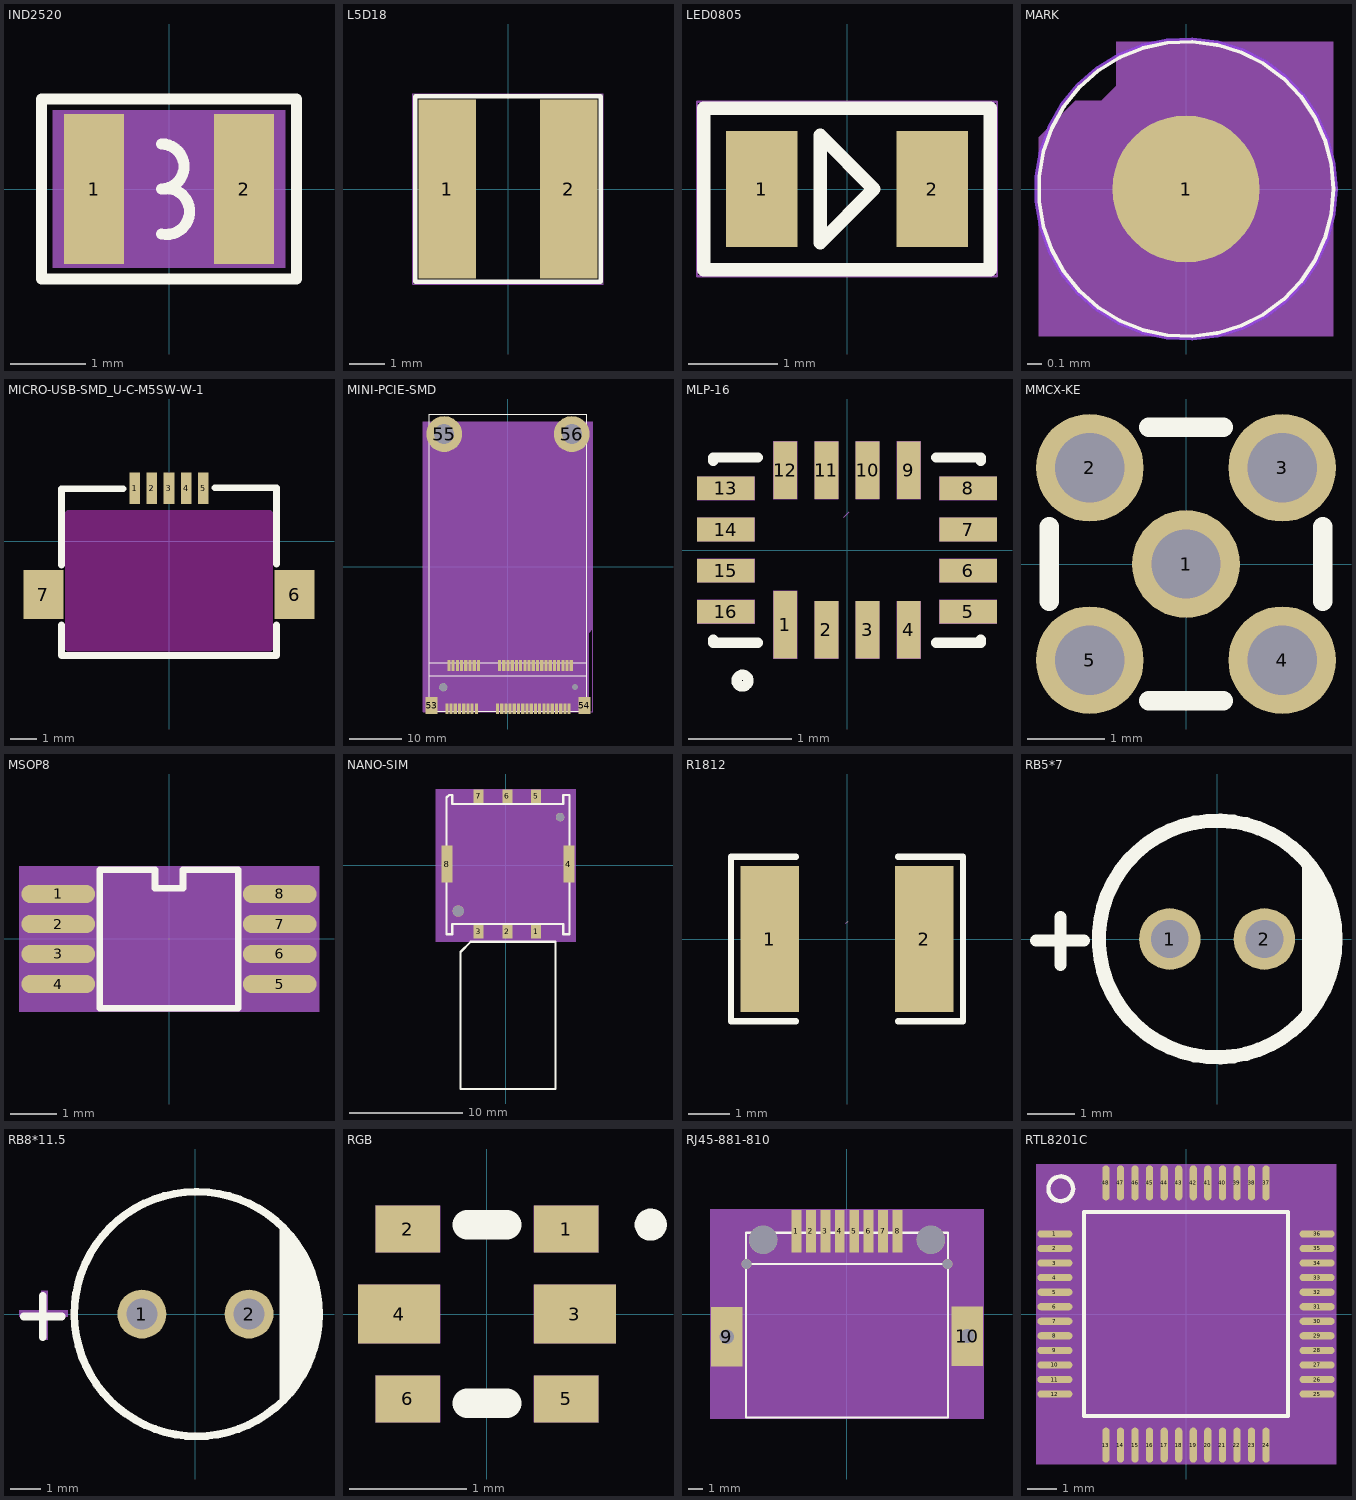
[diagram p0: the footprints below, top view; thin cyan lines are the x and y axes]
# Altium footprint library MISC84456-5.PcbLib: 85 footprints (part 3 of 6)
Each footprint in its own frame and in the unit in brackets; x right, y up, seen from the top. Pads: shape width x height; smd on the part's side, far side on the other; paste and mask are expansions set on the pad; w line width, h text height; cw(c..) or ccw(c..) is an arc to the next point about the centre after c.

## IND2520 [mm] "IND2520"
pads (2):
  rect 0.8x2 smd: 1(-1,0) 2(1,0)
Top Overlay:
  lines w0.15: -0.1,-0.6 ccw(c-0.033,-0.3) -0.1,0 ccw(c-0.1,0.3) -0.1,0.6 ; -1.7,-1.2 -1.7,0.4 -1.7,1.2 1.7,1.2 1.7,-1.2 -1.7,-1.2
Mechanical 7:
  text "2" at 1,-0.254 h0.64
  text "1" at -1,-0.254 h0.64
Mechanical 8:
  region: -1.55,1.05 -1.55,-1.05 1.55,-1.05 1.55,1.05
Mechanical 9:
  text "3.3uH" at 0.25,-0.75 h0.35
  text ".Designator" at 0.2,-0.525 h0.35

## L5D18 [mm] "L5D18"
pads (2):
  rect 1.6x5 smd: 1(-1.7,0) 2(1.7,0)
Top Overlay:
  lines w0.127: -2.6,-2.6 2.6,-2.6 2.6,2.6 -2.6,2.6 -2.6,-2.6
Mechanical 7:
  text "1" at -1.954,0 h0.64
  text "2" at 1.446,0 h0.64
Mechanical 8:
  lines w0.025: -2.663,-2.663 2.663,-2.663 2.663,2.663 -2.663,2.663 -2.663,-2.663
Mechanical 9:
  text "2.2uH/5x5" at -1.6,0.225 h0.35
  text ".Designator" at -0.2,0.625 h0.35

## LED0805 [mm] "LED0805"
pads (2):
  rect 0.8x1.3 smd: 1(-0.95,0) 2(0.95,0)
Top Overlay:
  lines w0.15: -1.6,-0.9 -1.6,0.9 -0.4,0.9 1.6,0.9 1.6,-0.9 -1.6,-0.9 ; -0.3,-0.6 -0.3,0.6 0.3,0 -0.3,-0.6
Mechanical 7:
  text "2" at 0.696,0 h0.64
  text "1" at -1.204,0 h0.64
Mechanical 8:
  lines w0.025: -1.675,-0.975 1.675,-0.975 1.675,0.975 -1.675,0.975 -1.675,-0.975
Mechanical 9:
  text "GREEN" at -0.925,-0.15 h0.35
  text ".Designator" at -0.32,-0.125 h0.35

## MARK [mm] "MARK"
pads (1):
  round 1 smd: 1(0,0)
Top Layer keep-out:
  circle w0.025: c0,0 r1.018
Bottom Layer keep-out:
  circle w0.025: c0,0 r1.018
Top Overlay:
  circle w0.025: c0,0 r1.001
Mechanical 7:
  text "1" at -0.254,0 h0.64
Mechanical 8:
  region: -1.001,-1.001 1.001,-1.001 1.001,1.001 -0.475,1.001 -0.475,0.7 -0.575,0.6 -0.751,0.6 -1.001,0.35

## MICRO-USB-SMD_U-C-M5SW-W-1 [mm]
pads (7):
  rect 0.4x1.2 smd: 1(-1.3,2.01) 2(-0.65,2.01) 3(0,2.01) 4(0.65,2.01) 5(1.3,2.01)
  rect 1.5x1.85 smd: 6(4.75,-2.01) 7(-4.75,-2.01)
Top Overlay:
  lines w0.254: -4.064,-3.175 -4.064,-3.165 -4.064,-4.318 4.064,-4.318 4.064,-3.165 4.064,-3.175 ; -4.064,-0.889 -4.064,1.997 -1.731,1.997 ; 1.732,2.032 4.064,2.032 4.064,-0.854 4.064,-0.762
Keep-Out Layer:
  board cut-out: -3.81,1.04 3.81,1.04 3.8,-4.04 -3.8,-4.04
  lines w0.254: -3.8,-4.04 -3.8,1.06 3.8,1.06 3.8,-4.04 -3.8,-4.04

## MINI-PCIE-SMD [mm] "MINI-PCIE-SMD"
pads (58):
  rect 0.6x2 smd: 1(-11.6,-26.925) 2(-11.2,-18.725) 3(-10.8,-26.925) 4(-10.4,-18.725) 5(-10,-26.925) 6(-9.6,-18.725) 7(-9.2,-26.925) 8(-8.8,-18.725) 9(-8.4,-26.925) 10(-8,-18.725) 11(-7.6,-26.925) 12(-7.2,-18.725) 13(-6.8,-26.925) 14(-6.4,-18.725) 15(-6,-26.925) 16(-5.6,-18.725) 17(-2,-26.925) 18(-1.6,-18.725) 19(-1.2,-26.925) 20(-0.8,-18.725) 21(-0.4,-26.925) 22(0,-18.725) 23(0.4,-26.925) 24(0.8,-18.725) 25(1.2,-26.925) 26(1.6,-18.725) 27(2,-26.925) 28(2.4,-18.725) 29(2.8,-26.925) 30(3.2,-18.725) 31(3.6,-26.925) 32(4,-18.725) 33(4.4,-26.925) 34(4.8,-18.725) 35(5.2,-26.925) 36(5.6,-18.725) 37(6,-26.925) 38(6.4,-18.725) 39(6.8,-26.925) 40(7.2,-18.725) 41(7.6,-26.925) 42(8,-18.725) 43(8.4,-26.925) 44(8.8,-18.725) 45(9.2,-26.925) 46(9.6,-18.725) 47(10,-26.925) 48(10.4,-18.725) 49(10.8,-26.925) 50(11.2,-18.725) 51(11.6,-26.925) 52(12,-18.725)
  rect 2.3x3.2 smd: 53(-14.5,-26.325) 54(14.5,-26.325)
  round 6.8 hole 3.8: 55(-12.1,25.175) 56(12.1,25.175)
  round 0.6 hole 1.6: " "(-12.3,-22.825)
  round 0.1 hole 1.1: " "(12.7,-22.825)
Top Overlay:
  lines w0.127: -14.95,-27.425 -14.95,-18.225 14.95,-18.225 14.95,-27.425 -14.95,-27.425
  lines w0.2: -14.9,-20.625 14.9,-20.625 14.9,28.975 -14.9,28.975 -14.9,-20.625
Mechanical 7:
  text "10" at -7.492,-18.725 h0.64
  text "2" at -10.946,-18.725 h0.64
  text "52" at 12.508,-18.725 h0.64
  text "41" at 8.108,-26.925 h0.64
  text "39" at 7.308,-26.925 h0.64
  text "14" at -5.892,-18.725 h0.64
  text "12" at -6.692,-18.725 h0.64
  text "8" at -8.546,-18.725 h0.64
  text "38" at 6.908,-18.725 h0.64
  text "36" at 6.108,-18.725 h0.64
  text "56" at 12.608,25.175 h0.64
  text "55" at -11.592,25.175 h0.64
  text "26" at 2.108,-18.725 h0.64
  text "34" at 5.308,-18.725 h0.64
  text "40" at 7.708,-18.725 h0.64
  text "21" at 0.108,-26.925 h0.64
  text "27" at 2.508,-26.925 h0.64
  text "29" at 3.308,-26.925 h0.64
  text "35" at 5.708,-26.925 h0.64
  text "37" at 6.508,-26.925 h0.64
  text "43" at 8.908,-26.925 h0.64
  text "54" at 15.008,-26.325 h0.64
  text "50" at 11.708,-18.725 h0.64
  text "4" at -10.146,-18.725 h0.64
  text "53" at -13.992,-26.325 h0.64
  text "9" at -8.146,-26.925 h0.64
  text "15" at -5.492,-26.925 h0.64
  text "18" at -1.092,-18.725 h0.64
  text "46" at 10.108,-18.725 h0.64
  text "44" at 9.308,-18.725 h0.64
  text "30" at 3.708,-18.725 h0.64
  text "32" at 4.508,-18.725 h0.64
  text "13" at -6.292,-26.925 h0.64
  text "11" at -7.092,-26.925 h0.64
  text "25" at 1.708,-26.925 h0.64
  text "17" at -1.492,-26.925 h0.64
  text "31" at 4.108,-26.925 h0.64
  text "33" at 4.908,-26.925 h0.64
  text "23" at 0.908,-26.925 h0.64
  text "24" at 1.308,-18.725 h0.64
  text "20" at -0.292,-18.725 h0.64
  text "16" at -5.092,-18.725 h0.64
  text "6" at -9.346,-18.725 h0.64
  text "48" at 10.908,-18.725 h0.64
  text "28" at 2.908,-18.725 h0.64
  text "19" at -0.692,-26.925 h0.64
  text "22" at 0.508,-18.725 h0.64
  text "51" at 12.108,-26.925 h0.64
  text "47" at 10.508,-26.925 h0.64
  text "49" at 11.308,-26.925 h0.64
  text "45" at 9.708,-26.925 h0.64
  text "1" at -11.346,-26.925 h0.64
  text "3" at -10.546,-26.925 h0.64
  text "42" at 8.508,-18.725 h0.64
  text "5" at -9.746,-26.925 h0.64
  text "7" at -8.946,-26.925 h0.64
Mechanical 8:
  region: -16.1,-27.475 15.275,-27.475 15.275,-12.6 16.1,-11.775 16.1,27.475 -16.1,27.475
Mechanical 9:
  lines w0.025: -16.1,-27.475 16.1,-27.475 16.1,27.475 -16.1,27.475 -16.1,-27.475
  text ".Designator" at -3.55,-24.425 h0.35

## MLP-16 [mm]
pads (16):
  rect 0.23x0.66 smd: 1(-0.6,-0.726)
  rect 0.23x0.56 smd: 2(-0.2,-0.776) 3(0.2,-0.776) 4(0.6,-0.776) 9(0.6,0.776) 10(0.2,0.776) 11(-0.2,0.776) 12(-0.6,0.776)
  rect 0.56x0.23 smd: 5(1.179,-0.6) 6(1.179,-0.2) 7(1.179,0.2) 8(1.179,0.6) 13(-1.179,0.6) 14(-1.179,0.2) 15(-1.179,-0.2) 16(-1.179,-0.6)
Top Overlay:
  circle w0.1: c-1.016,-1.27 r0.057
  lines w0.1: -1.3,-0.869 -1.3,-0.9 -0.869,-0.9 ; -1.3,0.869 -1.3,0.9 -0.869,0.9 ; 0.869,-0.9 1.3,-0.9 1.3,-0.869 ; 0.869,0.9 1.3,0.9 1.3,0.869
Mechanical 5:
  region: -1.459,0.715 -0.899,0.715 -0.899,0.485 -1.459,0.485
  region: -1.459,0.315 -0.899,0.315 -0.899,0.085 -1.459,0.085
  region: -1.459,-0.085 -0.899,-0.085 -0.899,-0.315 -1.459,-0.315
  region: -1.459,-0.485 -0.899,-0.485 -0.899,-0.715 -1.459,-0.715
  region: 0.485,1.056 0.715,1.056 0.715,0.496 0.485,0.496
  region: 0.085,1.056 0.315,1.056 0.315,0.496 0.085,0.496
  region: -0.315,1.056 -0.085,1.056 -0.085,0.496 -0.315,0.496
  region: -0.715,1.056 -0.485,1.056 -0.485,0.496 -0.715,0.496
  region: 0.899,0.715 1.459,0.715 1.459,0.485 0.899,0.485
  region: 0.899,0.315 1.459,0.315 1.459,0.085 0.899,0.085
  region: 0.899,-0.085 1.459,-0.085 1.459,-0.315 0.899,-0.315
  region: 0.899,-0.485 1.459,-0.485 1.459,-0.715 0.899,-0.715
  region: 0.485,-0.496 0.715,-0.496 0.715,-1.056 0.485,-1.056
  region: 0.085,-0.496 0.315,-0.496 0.315,-1.056 0.085,-1.056
  region: -0.315,-0.496 -0.085,-0.496 -0.085,-1.056 -0.315,-1.056
  region: -0.715,-0.396 -0.485,-0.396 -0.485,-1.056 -0.715,-1.056
Mechanical 15:
  lines w0.003: -0.03,0.321 0.021,0.372

## MMCX-KE [mm]
pads (5):
  round 1.4 hole 0.9: 1(0,0) 2(-1.25,1.25) 3(1.25,1.25) 4(1.25,-1.25) 5(-1.25,-1.25)
Top Overlay:
  lines w0.254: -1.778,-0.484 -1.778,0.484 ; -0.484,-1.778 0.484,-1.778 ; -0.484,1.778 0.484,1.778 ; 1.778,-0.484 1.778,0.484
Mechanical 15:
  lines w0.003: -0.025,0.492 0.025,0.543

## MSOP8 [mil] "MSOP8"
pads (8):
  oval 63x15.7 smd: 1(-94.5,38.4) 2(-94.5,12.8) 3(-94.5,-12.8) 4(-94.5,-38.4) 5(94.5,-38.4) 6(94.5,-12.8) 7(94.5,12.8) 8(94.5,38.4)
Top Overlay:
  lines w5.9: -59.1,-59.1 59.1,-59.1 59.1,59.1 11.8,59.1 11.8,43.3 -11.8,43.3 -11.8,59.1 -59.1,59.1 -59.1,-59.1
Mechanical 7:
  text "2" at -84.5,12.8 h25
  text "1" at -84.5,38.4 h25
  text "8" at 104.5,38.4 h25
  text "6" at 104.5,-12.8 h25
  text "5" at 104.5,-38.4 h25
  text "4" at -84.5,-38.4 h25
  text "3" at -84.5,-12.8 h25
  text "7" at 104.5,12.8 h25
Mechanical 8:
  region: -128,-62 128,-62 128,62 -128,62
Mechanical 9:
  text "HYM8563" at 49.21,4.92 h13.78
  text ".Designator" at 31.5,-16.73 h13.78

## NANO-SIM [mm] "NANO-SIM"
pads (10):
  rect 0.9x1.2 smd: 1(2.68,-5.85) 2(0.14,-5.85) 3(-2.4,-5.85) 5(2.68,6.1) 6(0.14,6.1) 7(-2.4,6.1)
  rect 1x3.3 smd: 4(5.58,0.12) 8(-5.19,0.12)
  round 1 hole 1: " "(-4.2,-4.03)
  round 0.75 hole 0.75: " "(4.8,4.27)
Top Overlay:
  lines w0.2: -5.23,-6.075 -5.23,5.995 -5,6.225 -4.725,6.225 -4.725,5.425 5.07,5.425 5.07,6.225 5.62,6.225 5.62,-6.075 5.07,-6.075 5.07,-5.175 -4.725,-5.175 -4.725,-6.075 -5.23,-6.075 ; -4,-19.75 4.4,-19.75 4.4,-6.75 -3.1,-6.75 -4,-7.65 -4,-19.75
  text ".Designator" at -6.45,-4.9 h0.6
Mechanical 7:
  text "7" at -2.146,6.1 h0.64
  text "2" at 0.394,-5.85 h0.64
  text "3" at -2.146,-5.85 h0.64
  text "1" at 2.934,-5.85 h0.64
  text "8" at -4.682,0.12 h0.64
  text "4" at 6.088,0.12 h0.64
  text "5" at 2.934,6.1 h0.64
  text "6" at 0.394,6.1 h0.64
Mechanical 8:
  region: -6.2,6.75 -6.2,-6.75 6.2,-6.75 6.2,6.75

## R1812 [mm]
pads (2):
  rect 1.407x3.499 smd: 1(-1.853,0) 2(1.853,0)
Top Overlay:
  lines w0.152: -1.226,-1.978 -2.785,-1.978 -2.785,1.978 -1.226,1.978 ; 1.226,-1.978 2.785,-1.978 2.785,1.978 1.226,1.978
Top Paste:
  region: 1.15,-1.65 1.15,-0.695 1.25,-0.595 1.528,-0.595 1.628,-0.495 1.628,0.495 1.528,0.595 1.25,0.595 1.15,0.695 1.15,1.65 1.25,1.75 2.457,1.75 2.557,1.65 2.557,-1.65 2.457,-1.75 1.25,-1.75
  region: -1.15,-1.65 -1.15,-0.695 -1.25,-0.595 -1.528,-0.595 -1.628,-0.495 -1.628,0.495 -1.528,0.595 -1.25,0.595 -1.15,0.695 -1.15,1.65 -1.25,1.75 -2.457,1.75 -2.557,1.65 -2.557,-1.65 -2.457,-1.75 -1.25,-1.75
Mechanical 5:
  region: -2.275,-1.62 -2.275,1.62 -1.525,1.62 -1.525,-1.62
  region: 2.275,-1.62 2.275,1.62 1.525,1.62 1.525,-1.62
Mechanical 6:
  circle w0.06: c-2.275,-1.62 r0.03
Mechanical 15:
  lines w0.003: -0.025,0.376 0.025,0.427

## RB5*7 [mm]
pads (2):
  round 1.3 hole 0.8: 1(-1,0) 2(1,0)
Top Overlay:
  circle w0.3: c0,0 r2.5
  region: 1.799,1.656 1.839,1.622 2.124,1.275 2.336,0.878 2.467,0.448 2.511,0 2.467,-0.448 2.336,-0.878 2.124,-1.275 1.839,-1.622 1.799,-1.656 1.794,-1.651
  lines w0.254: -3.826,-0.036 -2.81,-0.036 ; -3.31,-0.552 -3.31,0.464
Mechanical 5:
  circle w0.3: c1,0 r0.15
  circle w0.3: c-1,0 r0.15

## RB8*11.5 [mm]
pads (2):
  round 1.6 hole 1: 1(-1.75,0) 2(1.75,0)
Top Overlay:
  region: 2.753,-3.003 3.059,-2.654 3.375,-2.18 3.628,-1.668 3.811,-1.128 3.922,-0.569 3.959,0 3.922,0.569 3.811,1.128 3.628,1.668 3.375,2.18 3.059,2.654 2.753,3.003 2.75,3
  lines w0.254: -5.615,-0.085 -4.37,-0.085 ; -4.992,-0.758 -4.992,0.588 ; 0.003,4 ccw(c0.038,0.001) 0.074,4
Mechanical 5:
  circle w0.3: c1.75,0 r0.15
  circle w0.3: c-1.75,0 r0.15
Mechanical 15:
  region: -5.77,0.115 -4.17,0.115 -4.17,-0.085 -5.77,-0.085
  region: -5.035,-0.84 -5.035,0.76 -4.835,0.76 -4.835,-0.84

## RGB [mm]
pads (6):
  rect 0.55x0.4 smd: 1(0.675,0.725) 2(-0.675,0.725) 5(0.675,-0.725) 6(-0.675,-0.725)
  rect 0.7x0.5 smd: 3(0.75,0) 4(-0.75,0)
Top Overlay:
  circle w0.15: c1.397,0.762 r0.062
  lines w0.254: -0.169,-0.762 0.169,-0.762 ; -0.169,0.762 0.169,0.762
Mechanical 5:
  region: 0.4,0.925 0.95,0.925 0.95,0.525 0.4,0.525
  region: -0.95,0.925 -0.4,0.925 -0.4,0.525 -0.95,0.525
  region: 0.4,0.25 1.1,0.25 1.1,-0.25 0.4,-0.25
  region: -1.1,0.25 -0.4,0.25 -0.4,-0.25 -1.1,-0.25
  region: 0.4,-0.525 0.95,-0.525 0.95,-0.925 0.4,-0.925
  region: -0.95,-0.525 -0.4,-0.525 -0.4,-0.925 -0.95,-0.925

## RJ45-881-810 [mm] "RJ45-881-810"
pads (14):
  rect 0.7x3 smd: 1(-3.57,5.838) 2(-2.55,5.838) 3(-1.53,5.838) 4(-0.51,5.838) 5(0.51,5.838) 6(1.53,5.838) 7(2.55,5.838) 8(3.57,5.838)
  rect 2.2x4.2 hole 1: 9(-8.5,-1.612) 10(8.5,-1.562)
  round 0.7 hole 0.7: " "(-7.1,3.538) " "(7.1,3.538)
  round 2 hole 2: " "(-5.925,5.238) " "(5.925,5.238)
Top Overlay:
  lines w0.15: -7,3.538 7,3.538 ; -7.15,-7.312 7.15,-7.312 7.15,5.738 -7.15,5.738 -7.15,-7.312
Mechanical 7:
  text "9" at -8.439,-1.612 h0.08
  text "7" at 2.611,5.838 h0.08
  text "8" at 3.631,5.838 h0.08
  text "5" at 0.571,5.838 h0.08
  text "4" at -0.449,5.838 h0.08
  text "1" at -3.509,5.838 h0.08
  text "10" at 8.622,-1.562 h0.08
  text "6" at 1.591,5.838 h0.08
  text "2" at -2.489,5.838 h0.08
  text "3" at -1.469,5.838 h0.08
Mechanical 8:
  region: -9.65,-7.387 9.65,-7.387 9.65,7.388 -9.65,7.388
Mechanical 9:
  text ".Designator" at 0.825,7.938 h0.35

## RTL8201C [mm] "RTL8201C"
pads (48):
  oval 1.2x0.25 smd: 1(-4.5,2.75) 2(-4.5,2.25) 3(-4.5,1.75) 4(-4.5,1.25) 5(-4.5,0.75) 6(-4.5,0.25) 7(-4.5,-0.25) 8(-4.5,-0.75) 9(-4.5,-1.25) 10(-4.5,-1.75) 11(-4.5,-2.25) 12(-4.5,-2.75) 25(4.5,-2.75) 26(4.5,-2.25) 27(4.5,-1.75) 28(4.5,-1.25) 29(4.5,-0.75) 30(4.5,-0.25) 31(4.5,0.25) 32(4.5,0.75) 33(4.5,1.25) 34(4.5,1.75) 35(4.5,2.25) 36(4.5,2.75)
  oval 0.25x1.2 smd: 13(-2.75,-4.5) 14(-2.25,-4.5) 15(-1.75,-4.5) 16(-1.25,-4.5) 17(-0.75,-4.5) 18(-0.25,-4.5) 19(0.25,-4.5) 20(0.75,-4.5) 21(1.25,-4.5) 22(1.75,-4.5) 23(2.25,-4.5) 24(2.75,-4.5) 37(2.75,4.5) 38(2.25,4.5) 39(1.75,4.5) 40(1.25,4.5) 41(0.75,4.5) 42(0.25,4.5) 43(-0.25,4.5) 44(-0.75,4.5) 45(-1.25,4.5) 46(-1.75,4.5) 47(-2.25,4.5) 48(-2.75,4.5)
Top Overlay:
  circle w0.15: c-4.3,4.3 r0.424
  lines w0.15: -3.5,-3.5 -3.5,3.5 3.5,3.5 3.5,-3.5 -3.5,-3.5
Mechanical 7:
  text "27" at 4.906,-1.75 h0.51
  text "29" at 4.906,-0.75 h0.51
  text "35" at 4.906,2.25 h0.51
  text "45" at -0.844,4.5 h0.51
  text "17" at -0.344,-4.5 h0.51
  text "11" at -4.094,-2.25 h0.51
  text "44" at -0.344,4.5 h0.51
  text "6" at -4.297,0.25 h0.51
  text "43" at 0.156,4.5 h0.51
  text "46" at -1.344,4.5 h0.51
  text "36" at 4.906,2.75 h0.51
  text "34" at 4.906,1.75 h0.51
  text "1" at -4.297,2.75 h0.51
  text "37" at 3.156,4.5 h0.51
  text "2" at -4.297,2.25 h0.51
  text "30" at 4.906,-0.25 h0.51
  text "3" at -4.297,1.75 h0.51
  text "12" at -4.094,-2.75 h0.51
  text "32" at 4.906,0.75 h0.51
  text "41" at 1.156,4.5 h0.51
  text "4" at -4.297,1.25 h0.51
  text "39" at 2.156,4.5 h0.51
  text "9" at -4.297,-1.25 h0.51
  text "21" at 1.656,-4.5 h0.51
  text "20" at 1.156,-4.5 h0.51
  text "31" at 4.906,0.25 h0.51
  text "42" at 0.656,4.5 h0.51
  text "48" at -2.344,4.5 h0.51
  text "14" at -1.844,-4.5 h0.51
  text "26" at 4.906,-2.25 h0.51
  text "7" at -4.297,-0.25 h0.51
  text "8" at -4.297,-0.75 h0.51
  text "47" at -1.844,4.5 h0.51
  text "28" at 4.906,-1.25 h0.51
  text "10" at -4.094,-1.75 h0.51
  text "23" at 2.656,-4.5 h0.51
  text "16" at -0.844,-4.5 h0.51
  text "18" at 0.156,-4.5 h0.51
  text "19" at 0.656,-4.5 h0.51
  text "22" at 2.156,-4.5 h0.51
  text "13" at -2.344,-4.5 h0.51
  text "15" at -1.344,-4.5 h0.51
  text "25" at 4.906,-2.75 h0.51
  text "24" at 3.156,-4.5 h0.51
  text "38" at 2.656,4.5 h0.51
  text "5" at -4.297,0.75 h0.51
  text "33" at 4.906,1.25 h0.51
  text "40" at 1.656,4.5 h0.51
Mechanical 8:
  region: -5.15,-5.15 5.15,-5.15 5.15,5.15 -5.15,5.15
Mechanical 9:
  text ".Designator" at 0.57,-2.725 h0.35
  text "IP101A_RTL8201CP" at 2.825,-2.35 h0.35